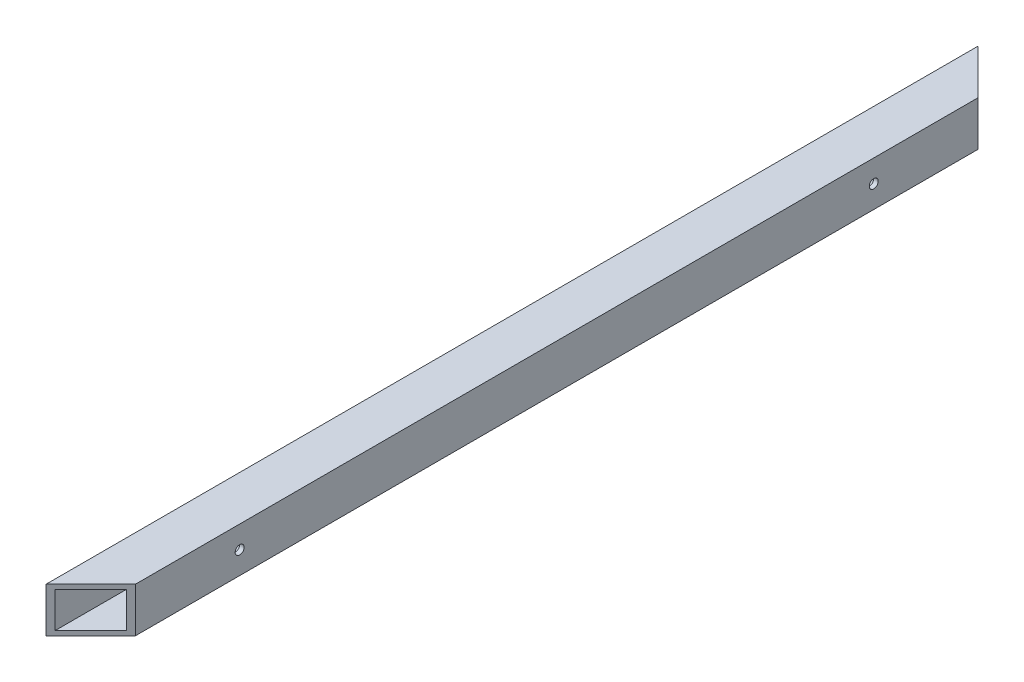
from build123d import *

# Parameters (mm, degrees)
SKETCH1_W           = 30
SKETCH1_H           = 30
BOSS_EXTRUDE1_DEPTH = 800
SKETCH2_W           = 24
SKETCH2_H           = 24
CUT_EXTRUDE1_DEPTH  = 800
CUT_EXTRUDE2_DEPTH  = 802.704175948
SKETCH4_R           = 3
CUT_EXTRUDE3_DEPTH  = 754.969037173


with BuildPart() as part:
    # Sketch1 → Boss-Extrude1 (new body)
    with BuildSketch(Plane.XY):
        with Locations((-27.773656986, 31.621806058)):
            Rectangle(SKETCH1_W, SKETCH1_H)
    extrude(amount=BOSS_EXTRUDE1_DEPTH)

    # Sketch2 → Cut-Extrude1 (cut)
    with BuildSketch(Plane.XY.offset(800)):
        with Locations((-27.773656986, 31.621806058)):
            Rectangle(SKETCH2_W, SKETCH2_H)
    extrude(amount=-CUT_EXTRUDE1_DEPTH, mode=Mode.SUBTRACT)

    # Sketch3 → Cut-Extrude2 (cut, through all)
    with BuildSketch(Plane(origin=(0, 16.621806058, 0), x_dir=(-1, 0, 0), z_dir=(0, -1, 0))):
        Polygon((12.773656986, -721.664630148), (42.773656986, -751.664630148), (42.773656986, -800), (12.773656986, -800), align=None)
        Polygon((12.773656986, -155.979205198), (42.773656986, -125.979205198), (42.773656986, 0), (12.773656986, 0), align=None)
    extrude(amount=-CUT_EXTRUDE2_DEPTH, mode=Mode.SUBTRACT)

    # Sketch4 → Cut-Extrude3 (cut, through all)
    with BuildSketch(Plane.ZY.offset(48.773656986)):
        with Locations(Location((225.979205198, 31.621806058, 0), (0, 0, 270))):
            Circle(SKETCH4_R)
        with Locations((225.979205198, 841.621806058)):
            Circle(SKETCH4_R)
        with Locations((651.664630148, 841.621806058)):
            Circle(SKETCH4_R)
        with Locations(Location((651.664630148, 31.621806058, 0), (0, 0, 269.999999999))):
            Circle(SKETCH4_R)
    extrude(amount=-CUT_EXTRUDE3_DEPTH, mode=Mode.SUBTRACT)


solid = part.part
